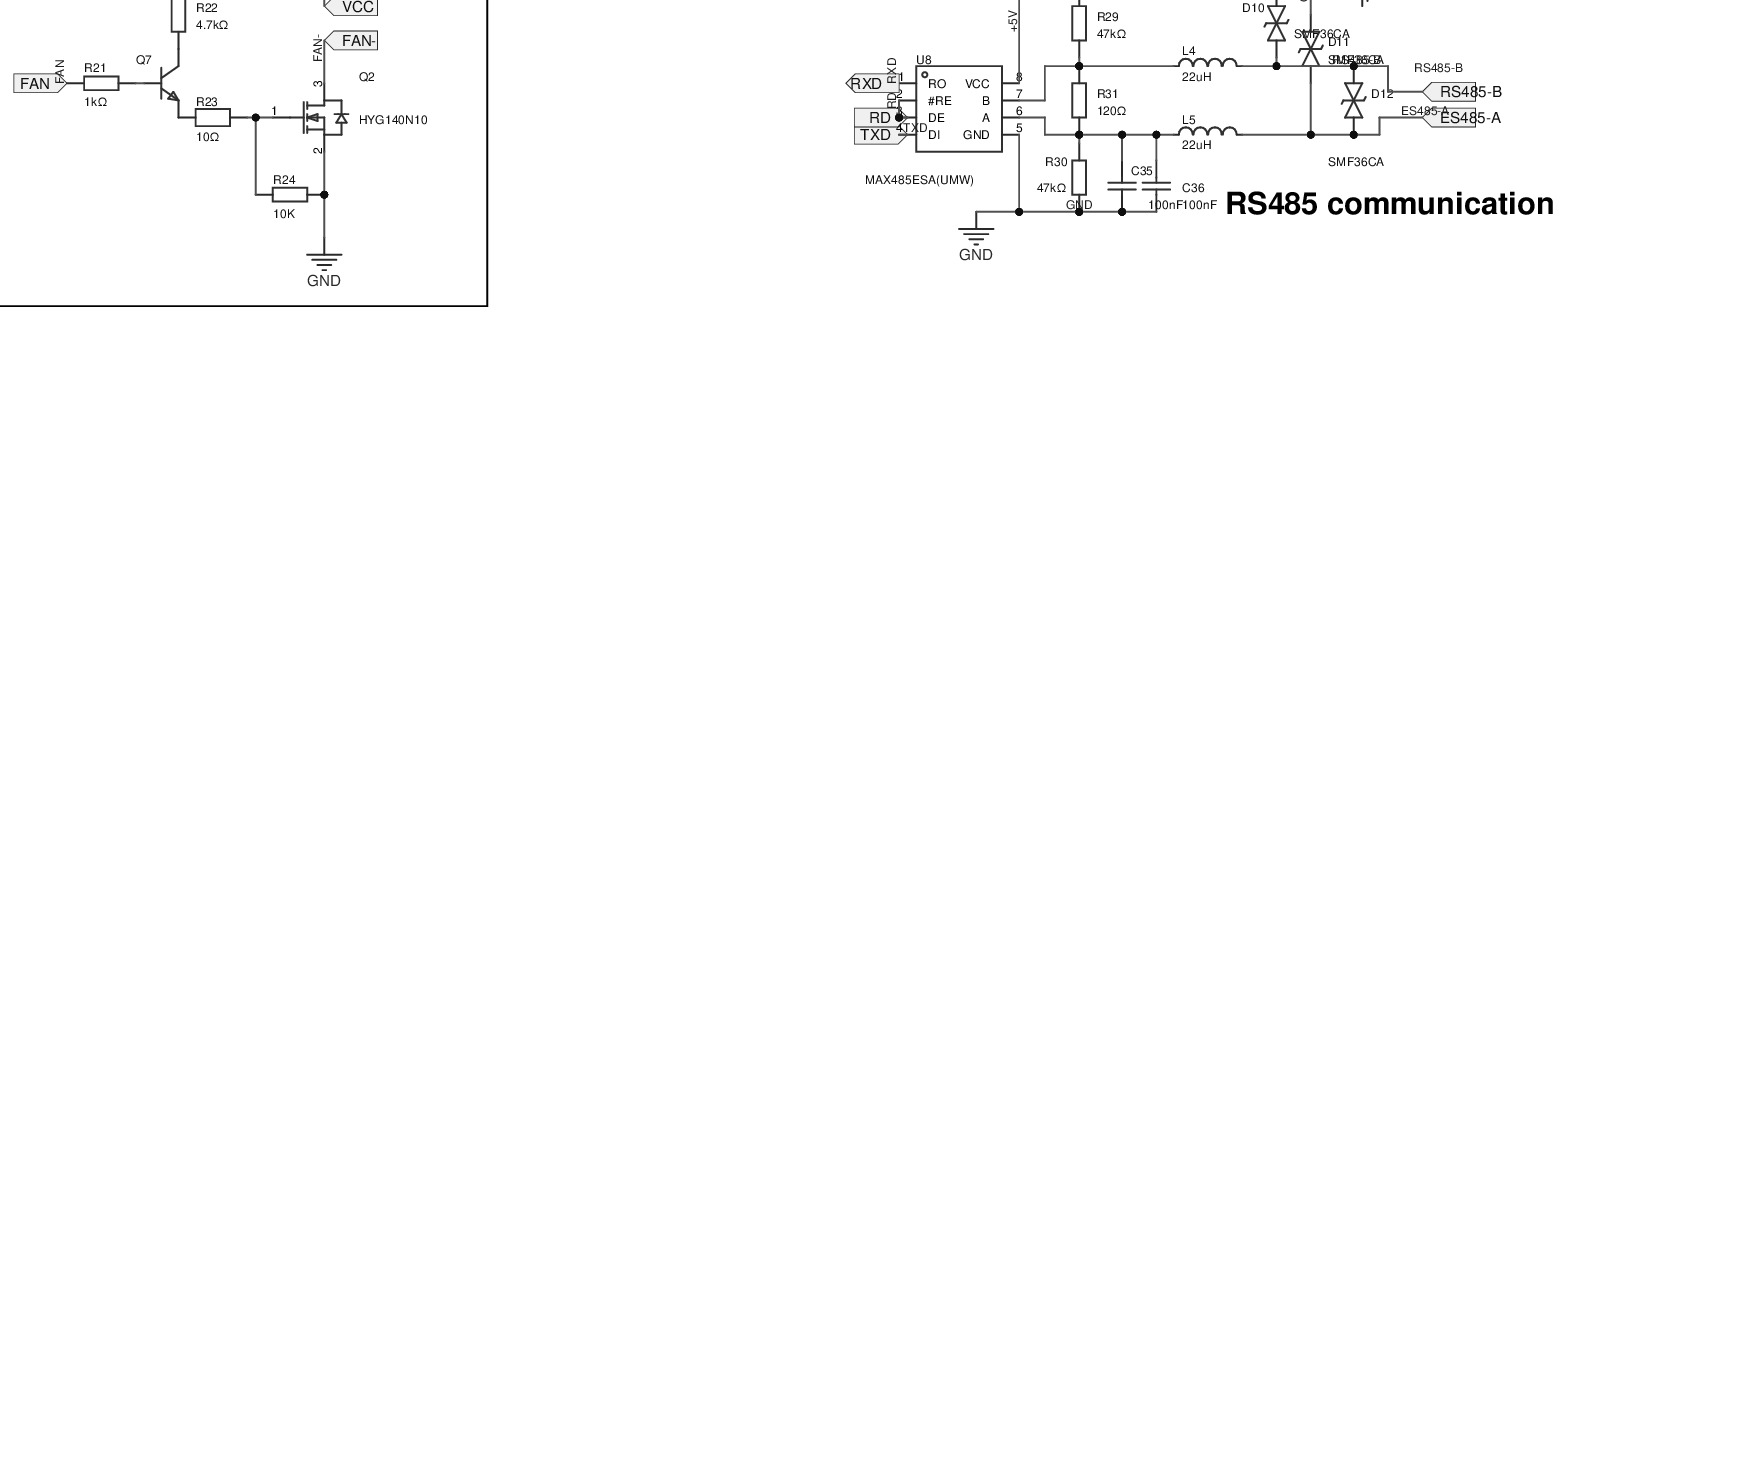
[diagram p0: MISC82093-2.schdoc, bottom right]
# Altium schematic sheet MISC82093-2.schdoc (part 2 of 2)

## Library data of the parts
BUZZER1 = YS-SBZ9650DYB05: Driving method: active (built-in driver circuit); frequency: 2.7kHz; sound pressure (SPL): 80dB;; Manufacturer: Fengming(锋鸣电子); Symbol: YS-SBZ9650DYB05_C409830; AddInBom: yes; ModelId: d9f071f9511e4f7795b1f85db8085480; ModelName: BUZ-SMD_L9.6-W9.6-H5.0; ModelTransform: 393.7,377.952,0,0,0,0,0,0,0; Voltage - Supply: 3V~7V; Device: YS-SBZ9650DYB05; LCSC Part Name: 贴片有源蜂鸣器5V; SupplierPart: C409830; ManufacturerPart: YS-SBZ9650DYB05; Supplier Footprint: SMD,9.6x9.6mm; JLCPCB Part Class: Extended library; Datasheet: https://item.szlcsc.com/datasheet/YS-SBZ9650DYB05/400193.html; Supplier: LCSC; ConvertToPcb: yes; FootprintName: BUZ-SMD_L9.6-W9.6-LS10.0-R; Driver Circuitry: Active (built-in driver circuit); Value: 2.7kHz; Sound Pressure Level(SPL): 80dB; Length: 9.6mm; Width: 9.6mm; Height: 5.3mm
C1 = ECF1KM330F12OTPO: Capacitance: 33uF; tolerance: ±20%; rated voltage: 100V; ripple current: -; equivalent series resistance (ESR): -;; Manufacturer: Yunxing(云星); AddInBom: yes; ModelId: 1445cc51bd6740cbb18bd7447caccb15; ModelTransform: 314.96,315.3537,0,90,0,0,0,0,-196.85; Lifetime: 6000hrs@105℃; Symbol: ECF1KM330F12OTPO; Device: ECF1KM330F12OTPO; LCSC Part Name: 33uF ±20% 100V; SupplierPart: C783507; ManufacturerPart: ECF1KM330F12OTPO; Supplier Footprint: 插件,D8xL12mm; JLCPCB Part Class: Extended library; Datasheet: https://item.szlcsc.com/datasheet/ECF1KM330F12OTPO/837832.html; Supplier: LCSC; ConvertToPcb: yes; FootprintName: CAP-TH_BD8.0-P3.50-D1.0-FD; ModelName: CAP-TH_BD8.0-P3.50-D1.0-FD; Value: 33uF; Tolerance: ±20%; Voltage Rating: 100V; Ripple Current: -; Equivalent Series Resistance(ESR): -; Pin Spacing: -; Diameter: 8mm; Height - Seated (Max): 12mm; Operating Temperature: -40℃~+105℃
C2 C3 = GRM31CL8EL225KE07L: Capacitance: 2.2uF; tolerance: ±10%; rated voltage: 100V; dielectric (temperature coefficient): X8L;; Manufacturer: muRata(村田); AddInBom: yes; ModelId: e4be705b945545a48e666415e3682bd8; ModelName: C1206_L3.2-W1.6-H1.3; ModelTransform: 125.984,62.992,0,0,0,0,0,0,0; Symbol: GRM31CL8EL225KE07L; Device: GRM31CL8EL225KE07L; LCSC Part Name: 2.2uF ±10% 100V; SupplierPart: C5119320; ManufacturerPart: GRM31CL8EL225KE07L; Supplier Footprint: 1206; JLCPCB Part Class: Extended library; Datasheet: https://atta.szlcsc.com/upload/public/pdf/source/20220725/4E0CF642079D992081E87782F4D32939.pdf; Supplier: LCSC; ConvertToPcb: yes; FootprintName: C1206; Value: 2.2uF; Tolerance: ±10%; Voltage Rated: 100V; Temperature Coefficient: X8L
C4 C5 = CAP_1206: Symbol: Capacitance; ConvertToPcb: yes; ModelId: e4be705b945545a48e666415e3682bd8; ModelName: C1206_L3.2-W1.6-H1.3; ModelTransform: 125.984,62.992,0,0,0,0,0,0,0; Device: CAP_1206; AddInBom: yes; Supplier Footprint: 1206; FootprintName: C1206
  C4: Value: 100nF
  C5: Value: 1nF
C6 C9 C10 C13 C14 C16-C19 C23-C26 C30 C35-C37 = CL21B104KBCNNNC: Capacitance: 100nF; tolerance: ±10%; rated voltage: 50V; temperature coefficient: X7R;; Manufacturer: SAMSUNG(三星); AddInBom: yes; ModelId: 1ba041120af144c991958decab20d2410819f05c4eef4c71ace90d822a990e87; ModelName: C0805_L2.0-W1.3-H1.3; ModelTransform: 78.74,51.181,0,0,0,0,0,0.0005,0; Symbol: CL21B104KBCNNNC; Device: CL21B104KBCNNNC; LCSC Part Name: 100nF ±10% 50V; SupplierPart: C1711; ManufacturerPart: CL21B104KBCNNNC; Supplier Footprint: 0805; JLCPCB Part Class: Extended Part; Datasheet: https://item.szlcsc.com/datasheet/CL21B104KBCNNNC/2063.html; Supplier: LCSC; ConvertToPcb: yes; FootprintName: C0805; Value: 100nF; Tolerance: ±10%; Voltage Rating: 50V; Temperature Coefficient: X7R
C7 = GRJ32EC71E226KE11L: Capacitance: 22uF; tolerance: ±10%; rated voltage: 25V; dielectric (temperature coefficient): X7S;; Manufacturer: muRata(村田); AddInBom: yes; ModelId: 833068e7fe044595a6eec77c56179455; ModelName: C1210_L3.2-W2.5-H2.5; ModelTransform: 125.984,98.425,0,0,0,0,0,0,0; Symbol: GRJ32EC71E226KE11L; Device: GRJ32EC71E226KE11L; LCSC Part Name: 22uF ±10% 25V; SupplierPart: C5646747; ManufacturerPart: GRJ32EC71E226KE11L; Supplier Footprint: 1210; JLCPCB Part Class: Extended library; Datasheet: https://atta.szlcsc.com/upload/public/pdf/source/20230811/978878A2AA1A844A6A0C1208031DF55A.pdf; Supplier: LCSC; ConvertToPcb: yes; FootprintName: C1210; Value: 22uF; Tolerance: ±10%; Voltage Rated: 25V; Temperature Coefficient: X7S
C8 C11 = JVS25V100M6X4: Capacitance: 100uF; tolerance: ±20%; rated voltage: 25V; ripple current: 54mA@120Hz;; Manufacturer: JIERR(捷而瑞); AddInBom: yes; Lifetime: 1000hrs@105℃; Symbol: JVS25V100M6X4; Device: JVS25V100M6X4; LCSC Part Name: 100uF ±20% 25V; SupplierPart: C51953404; ManufacturerPart: JVS25V100M6X4; Supplier Footprint: SMD,D6.3xL4.5mm; JLCPCB Part Class: Extended Part; Datasheet: https://item.szlcsc.com/datasheet/JVS25V100M6X4/54681529.html; Supplier: LCSC; ConvertToPcb: yes; FootprintName: CAP-SMD_BD6.3-L6.6-W6.6-LS7.3-FD_JVS25V100M6X4; Value: 100uF; Tolerance: ±20%; Voltage Rating: 25V; Ripple Current: 54mA@120Hz; Diameter: 6.3mm; Height - Seated (Max): 4.5mm; Operating Temperature: -55℃~+105℃
C12 = 35PX470MEFC10X12.5: Capacitance: 470uF; tolerance: ±20%; rated voltage: 35V; ripple current: 525mA@120Hz; equivalent series resistance: -;; Manufacturer: rubycon(红宝石); AddInBom: yes; ModelId: 6ce78ce5315348e095d700085da75e480819f05c4eef4c71ace90d822a990e87; ModelName: CAP-TH_D10.0-H16.0-P5.00; ModelTransform: 394.094,393.72252,0,0,0,0,0,0,-137.795; φD: 10mm; L: 12.5mm; Lifetime @ Temp: 2000hrs@105℃; Symbol: 35PX470MEFC10X12.5; Device: 35PX470MEFC10X12.5; LCSC Part Name: 470uF ±20% 35V; SupplierPart: C127917; ManufacturerPart: 35PX470MEFC10X12.5; Supplier Footprint: 插件,D10xL12.5mm; JLCPCB Part Class: Extended Part; Datasheet: https://atta.szlcsc.com/upload/public/pdf/source/20171026/C136025_15089841766351059112.pdf; Supplier: LCSC; ConvertToPcb: yes; FootprintName: CAP-TH_BD10.0-P5.00-D1.0-FD; Value: 470uF; Tolerance: ±20%; Rated Voltage: 35V; Ripple Current: 525mA@120Hz; Equivalent Series Resistance(ESR): -; Lead Spacing: 5mm; Operating Temperature: -25℃~+105℃
C15 = JVS25V100M6X4: Capacitance: 100uF; tolerance: ±20%; rated voltage: 25V; ripple current: 54mA@120Hz;; Manufacturer: JIERR(捷而瑞); Lifetime: 1000hrs@105℃; AddInBom: yes; Symbol: JVS25V100M6X4; Device: JVS25V100M6X4; LCSC Part Name: 100uF ±20% 25V; Supplier Part: C51953404; Manufacturer Part: JVS25V100M6X4; Supplier Footprint: SMD,D6.3xL4.5mm; JLCPCB Part Class: Extended Part; Datasheet: https://item.szlcsc.com/datasheet/JVS25V100M6X4/54681529.html; Supplier: LCSC; Value: 100uF; Tolerance: ±20%; Voltage Rating: 25V; Ripple Current: 54mA@120Hz; Diameter: 6.3mm; Height - Seated (Max): 4.5mm; Operating Temperature: -55℃~+105℃; ConvertToPcb: yes; FootprintName: CAP-SMD_BD6.3-L6.6-W6.6-LS7.3-FD_JVS25V100M6X4
C20 = CAP_0805: Symbol: Capacitance; ConvertToPcb: yes; ModelId: 1ba041120af144c991958decab20d241; ModelName: C0805_L2.0-W1.3-H1.3; ModelTransform: 78.74,51.181,0,0,0,0,0,0.0005,0; Value: 0.1uF; Device: CAP_0805; AddInBom: yes; Supplier Footprint: 0805; FootprintName: C0805
C21 C22 = CL21C220JBANNNC: Capacitance: 22pF; tolerance: ±5%; rated voltage: 50V; temperature coefficient: C0G;; Manufacturer: SAMSUNG(三星); AddInBom: yes; ModelId: 1ba041120af144c991958decab20d2410819f05c4eef4c71ace90d822a990e87; ModelName: C0805_L2.0-W1.3-H1.3; ModelTransform: 78.74,51.181,0,0,0,0,0,0.0005,0; Symbol: CL21C220JBANNNC; Device: CL21C220JBANNNC; LCSC Part Name: 22pF ±5% 50V; SupplierPart: C1804; ManufacturerPart: CL21C220JBANNNC; Supplier Footprint: 0805; JLCPCB Part Class: Basic Part; Datasheet: https://item.szlcsc.com/datasheet/CL21C220JBANNNC/2156.html; Supplier: LCSC; ConvertToPcb: yes; FootprintName: C0805; Value: 22pF; Tolerance: ±5%; Voltage Rating: 50V; Temperature Coefficient: C0G
C27-C29 = CL21C101JBANNNC: Capacitance: 100pF; tolerance: ±5%; rated voltage: 50V; temperature coefficient: C0G;; Manufacturer: SAMSUNG(三星); AddInBom: yes; ModelId: 1ba041120af144c991958decab20d2410819f05c4eef4c71ace90d822a990e87; ModelName: C0805_L2.0-W1.3-H1.3; ModelTransform: 78.74,51.181,0,0,0,0,0,0.0005,0; Symbol: CL21C101JBANNNC; Device: CL21C101JBANNNC; LCSC Part Name: 100pF ±5% 50V; SupplierPart: C1790; ManufacturerPart: CL21C101JBANNNC; Supplier Footprint: 0805; JLCPCB Part Class: Basic Part; Datasheet: https://item.szlcsc.com/datasheet/CL21C101JBANNNC/2142.html; Supplier: LCSC; ConvertToPcb: yes; FootprintName: C0805; Value: 100pF; Tolerance: ±5%; Voltage Rating: 50V; Temperature Coefficient: C0G
C31-C34 = 0805X5R106K500NT: Capacitance: 10uF; tolerance: ±10%; rated voltage: 50V; temperature coefficient: X5R;; Manufacturer: AIDE(爱迪电容); AddInBom: yes; ModelId: 1ba041120af144c991958decab20d241; ModelName: C0805_L2.0-W1.3-H1.3; ModelTransform: 78.74,51.181,0,0,0,0,0,0.0005,0; Symbol: 0805X5R106K500NT; Device: 0805X5R106K500NT; LCSC Part Name: 10uF ±10% 50V; ManufacturerPart: 0805X5R106K500NT; Supplier Footprint: 0805; JLCPCB Part Class: Extended library; Datasheet: https://atta.szlcsc.com/upload/public/pdf/source/20250425/87F0660DBF100371164E520B4251C19E.pdf; Supplier: LCSC; ConvertToPcb: yes; FootprintName: C0805; Tolerance: ±10%; Voltage Rating: 50V; Temperature Coefficient: X5R
  C31 C33: SupplierPart: C48579582; Value: 10uF
  C32 C34: Value: 1uF
C38 C39 = GRJ32EC71E226KE11L: Capacitance: 22uF; tolerance: ±10%; rated voltage: 25V; dielectric (temperature coefficient): X7S;; Manufacturer: muRata(村田); 3D Model: 833068e7fe044595a6eec77c56179455; 3D Model Transform: 125.984,98.425,0,0,0,0,0,0,0; AddInBom: yes; ModelName: C1210_L3.2-W2.5-H2.5; Symbol: GRJ32EC71E226KE11L; Device: GRJ32EC71E226KE11L; LCSC Part Name: 22uF ±10% 25V; Supplier Part: C5646747; Manufacturer Part: GRJ32EC71E226KE11L; Supplier Footprint: 1210; JLCPCB Part Class: Extended library; Datasheet: https://atta.szlcsc.com/upload/public/pdf/source/20230811/978878A2AA1A844A6A0C1208031DF55A.pdf; Supplier: LCSC; Value: 22uF; Tolerance: ±10%; Voltage Rated: 25V; Temperature Coefficient: X7S; ConvertToPcb: yes; FootprintName: C1210
C40 = CL21B104KBCNNNC: Capacitance: 100nF; tolerance: ±10%; rated voltage: 50V; temperature coefficient: X7R;; Manufacturer: SAMSUNG(三星); 3D Model: 1ba041120af144c991958decab20d2410819f05c4eef4c71ace90d822a990e87; 3D Model Transform: 78.74,51.181,0,0,0,0,0,0.0005,0; AddInBom: yes; ModelName: C0805_L2.0-W1.3-H1.3; Symbol: CL21B104KBCNNNC; Device: CL21B104KBCNNNC; LCSC Part Name: 100nF ±10% 50V; Supplier Part: C1711; Manufacturer Part: CL21B104KBCNNNC; Supplier Footprint: 0805; JLCPCB Part Class: Extended Part; Datasheet: https://item.szlcsc.com/datasheet/CL21B104KBCNNNC/2063.html; Supplier: LCSC; Value: 100nF; Tolerance: ±10%; Voltage Rating: 50V; Temperature Coefficient: X7R; ConvertToPcb: yes; FootprintName: C0805
C41 = CL21B102KBCNNNC: Capacitance: 1nF; tolerance: ±10%; rated voltage: 50V; temperature coefficient: X7R;; Manufacturer: SAMSUNG(三星); AddInBom: yes; ModelId: 1ba041120af144c991958decab20d2410819f05c4eef4c71ace90d822a990e87; ModelName: C0805_L2.0-W1.3-H1.3; ModelTransform: 78.74,51.181,0,0,0,0,0,0.0005,0; Symbol: CL21B102KBCNNNC; Device: CL21B102KBCNNNC; LCSC Part Name: 1nF ±10% 50V; SupplierPart: C46653; ManufacturerPart: CL21B102KBCNNNC; Supplier Footprint: 0805; JLCPCB Part Class: Basic Part; Datasheet: https://item.szlcsc.com/datasheet/CL21B102KBCNNNC/47657.html; Supplier: LCSC; ConvertToPcb: yes; FootprintName: C0805; Value: 1nF; Tolerance: ±10%; Voltage Rating: 50V; Temperature Coefficient: X7R
D1 = US2M-TP: Diode configuration: -; forward voltage (Vf): 1.7V@2A; DC reverse voltage (Vr): 1kV; rectified current: 2A; reverse recovery time (Trr): 100ns;; Manufacturer: MCC(美微科); AddInBom: yes; ModelId: 5e8926c661484ff2a35b83e5ae62aeb90819f05c4eef4c71ace90d822a990e87; ModelTransform: 212.598,141.732,0,0,0,0,0,0,0; Reverse Leakage Current (Ir): 5uA@1kV; Operating Junction Temperature Range: -50℃~+150℃@(Ta); Non-Repetitive Peak Forward Surge Current: 50A; Symbol: US2M-TP; Device: US2M-TP; LCSC Part Name: 耐压:1kV 电流:2A 反向恢复时间：100ns; SupplierPart: C138791; ManufacturerPart: US2M-TP; Supplier Footprint: DO-214AA(SMB); JLCPCB Part Class: Extended Part; Datasheet: https://item.szlcsc.com/datasheet/US2M-TP/150112.html; Supplier: LCSC; ConvertToPcb: yes; FootprintName: SMB_L4.6-W3.6-LS5.3-RD; ModelName: SMB_L4.6-W3.6-LS5.3-RD; Diode Configuration: -; Voltage - Forward(Vf@If): 1.7V@2A; Voltage - DC Reverse(Vr): 1kV; Current - Rectified: 2A; Reverse Recovery Time (trr): 100ns
D2 D3 = SS34_C8678: Diode configuration: single; forward voltage (Vf): 550mV@3A; DC reverse voltage (Vr): 40V; rectified current: 3A;; Manufacturer: MDD(辰达半导体); 3D Model: e3551acb3c5a4975a5e9d36087fe1fa2; 3D Model Transform: 185.039,102.362,0,0,0,0,0,0,0; Reverse Leakage Current (Ir): 500uA@40V; Operating Junction Temperature Range: -55℃~+125℃; AddInBom: yes; Symbol: SS34_C8678; Device: SS34_C8678; LCSC Part Name: 电压:40V 电流:3A; Supplier Part: C8678; Manufacturer Part: SS34; Supplier Footprint: SMA(DO-214AC); JLCPCB Part Class: Basic library; Datasheet: https://item.szlcsc.com/datasheet/SS34/9178.html; Supplier: LCSC; Diode Configuration: Single; Voltage - Forward(Vf@If): 550mV@3A; Voltage - DC Reverse(Vr): 40V; Current - Rectified: 3A; ConvertToPcb: yes; FootprintName: SMA_L4.3-W2.6-LS5.2-RD; ModelName: SMA_L4.3-W2.6-LS5.2-RD
D4 D5 = MUR160SB: Diode configuration: single; forward voltage (Vf): 1.3V@1A; DC reverse voltage (Vr): 600V; rectified current: 1A; reverse recovery time (Trr): 50ns;; Manufacturer: AM(安美); AddInBom: yes; ModelId: 892cc756ed79448ab4afad0e5bfcdfa6; ModelTransform: 212.598,141.732,0,0,0,0,0,0,0; Symbol: MUR160SB; Device: MUR160SB; LCSC Part Name: MUR160SB; SupplierPart: C18336927; ManufacturerPart: MUR160SB; Supplier Footprint: SMB; JLCPCB Part Class: Extended library; Datasheet: https://atta.szlcsc.com/upload/public/pdf/source/20231016/5AD88B7244EB32ADD8FE31282D3178E2.pdf; Supplier: LCSC; ConvertToPcb: yes; FootprintName: SMB_L4.6-W3.6-LS5.3-RD; ModelName: SMB_L4.6-W3.6-LS5.3-RD; Diode Configuration: Single; Voltage - Forward(Vf@If): 1.3V@1A; Voltage - DC Reverse(Vr): 600V; Current - Rectified: 1A; Reverse Recovery Time (trr): 50ns
D6-D9 = RB160M-90: Forward voltage (Vf): 750mV@1.0A; DC reverse voltage (Vr): 90V; rectified current: 1A;; Manufacturer: TECH PUBLIC(台舟); AddInBom: yes; ModelId: 86f9151e155e4fe2af0c4f2e0a80302e; ModelName: SOD-123FL_L2.8-W1.8-H1.1-LS3.6; ModelTransform: 141.732,70.866,0,180,0,0,0,0,0; Reverse Leakage Current (Ir): 100uA@100V; Operating Junction Temperature Range: -55℃~+150℃; Non-Repetitive Peak Forward Surge Current: 50A; Symbol: RB160M-90; Device: RB160M-90; LCSC Part Name: 电压:90V 电流:1A; SupplierPart: C7603322; ManufacturerPart: RB160M-90; Supplier Footprint: SOD-123FL; JLCPCB Part Class: Extended library; Datasheet: https://item.szlcsc.com/datasheet/RB160M-90/8728828.html; Supplier: LCSC; ConvertToPcb: yes; FootprintName: SOD-123FL_L2.7-W1.8-LS3.7-RD; Voltage - Forward(Vf@If): 750mV@1.0A; Voltage - DC Reverse(Vr): 90V; Current - Rectified: 1A
D10-D12 = SMF36CA_C435502: Polarity: bidirectional; reverse standoff voltage (Vrwm): 36V; clamping voltage: 58.1V; peak pulse current (Ipp): 3.5A; peak pulse power (Ppp): 200W@10/1000us; breakdown voltage: 40V;; Manufacturer: AnBon(安邦); 3D Model: 8576f175c34f41329e79954aa68cc529; 3D Model Transform: 145.669,70.866,0,0,0,0,0,0,0; Reverse Leakage Current (Ir): 5uA; Number of Channels: Single channel; Type: TVS; AddInBom: yes; Symbol: SMF36CA_C435502; Device: SMF36CA_C435502; LCSC Part Name: SMF36CA; Supplier Part: C435502; Manufacturer Part: SMF36CA; Supplier Footprint: SOD-123; JLCPCB Part Class: Extended library; Datasheet: https://item.szlcsc.com/datasheet/SMF36CA/432840.html; Supplier: LCSC; Polarity: Bidirectional; Reverse Stand-Off Voltage (Vrwm): 36V; Clamping Voltage: 58.1V; Peak Pulse Current (Ipp): 3.5A; Peak Pulse Power Dissipation (Ppp): 200W@10/1000us; Voltage - Breakdown: 40V; Operating Temperature: -55℃~+150℃; ConvertToPcb: yes; FootprintName: SOD-123_L2.7-W1.8-LS3.7-BI; ModelName: SOD-123_L2.7-W1.8-LS3.7-BI
L1 = FXL1040-330-M: Inductance: 33uH; tolerance: ±20%; rated current: 4.4A; saturation current (Isat): 5A; type: molded inductor;; Manufacturer: cjiang(长江微电); 3D Model: c9cd86c9f1ef4d748cb9537bf0f243250819f05c4eef4c71ace90d822a990e87; 3D Model Transform: 452.755,393.7,0,0,0,0,0,0,0; DC Resistance(DCR): 92mΩ; AddInBom: yes; ModelName: IND-SMD_L11.5-W10.0-H3.8_FXL1040; Symbol: FXL1040-330-M; Device: FXL1040-330-M; LCSC Part Name: 33uH ±20% 5A; Supplier Part: C475918; Manufacturer Part: FXL1040-330-M; Supplier Footprint: SMD,11.5x10mm; JLCPCB Part Class: Extended Part; Datasheet: https://item.szlcsc.com/datasheet/FXL1040-330-M/482451.html; Supplier: LCSC; Value: 33uH; Tolerance: ±20%; Current Rating: 4.4A; Current - Saturation(Isat): 5A; Type: Molded inductor; ConvertToPcb: yes; FootprintName: IND-SMD_L11.5-W10.0_FXL1040
L2 L3 = PSPMAA0605H-680M-IGF: Inductance: 68uH; tolerance: ±20%; rated current: 1.5A; saturation current (Isat): 2A; type: -;; Manufacturer: PROD(谱罗德); AddInBom: yes; ModelId: 42305e89796f47b49312a685ea93d4940819f05c4eef4c71ace90d822a990e87; ModelName: IND-SMD_L7.1-W6.6-H5.0; ModelTransform: 275.59,259.88137,0,0,0,0,0,-0.551,0; DC Resistance(DCR): 256mΩ; Symbol: PSPMAA0605H-680M-IGF; Device: PSPMAA0605H-680M-IGF; LCSC Part Name: 68uH ±20% 2A; SupplierPart: C2983094; ManufacturerPart: PSPMAA0605H-680M-IGF; Supplier Footprint: SMD,7.1x6.6mm; JLCPCB Part Class: Extended Part; Datasheet: https://item.szlcsc.com/datasheet/PSPMAA0605H-680M-IGF/3416346.html; Supplier: LCSC; ConvertToPcb: yes; FootprintName: IND-SMD_L7.1-W6.6_H5.0; Value: 68uH; Tolerance: ±20%; Current Rating: 1.5A; Current - Saturation(Isat): 2A; Type: -; Ratings: -
L4 L5 = SCL3216T220KSP: Inductance: 22uH; tolerance: ±10%; rated current: 5mA; saturation current (Isat): -; DC resistance (DCR): 900mΩ;; Manufacturer: Sunltech(顺磁); AddInBom: yes; ModelId: 85bdab7b3d4c4074b81d208eb5e865b30819f05c4eef4c71ace90d822a990e87; ModelName: L1206_L3.2-W1.6-H1.1; ModelTransform: 125.984,62.835,0,0,0,0,0,0,0; Symbol: SCL3216T220KSP; Device: SCL3216T220KSP; LCSC Part Name: 22uH ±10%; SupplierPart: C412019; ManufacturerPart: SCL3216T220KSP; Supplier Footprint: 1206; JLCPCB Part Class: Extended Part; Datasheet: https://item.szlcsc.com/datasheet/SCL3216T220KSP/403512.html; Supplier: LCSC; ConvertToPcb: yes; FootprintName: L1206; Value: 22uH; Tolerance: ±10%; Current Rating: 5mA; Current - Saturation (Isat): -; DC Resistance(DCR): 900mΩ; Q @ Frequency: -; Frequency - Self Resonant: -; Ratings: -
LED1-LED4 = 3mmFIR: AddInBom: yes; ModelId: a497c992633541038a38947cdc58012f; ModelName: LED-TH-3mm_R; ModelTransform: 141.274,153.327,0,0,0,0,-5.984,0,-137.795; Symbol: 3MMFIR; Device: 3mmFIR; LCSC Part Name: 3mmFIR; SupplierPart: C9900095018; ManufacturerPart: 3mmFIR; Supplier Footprint: LED-TH_LED-3MM_RED; JLCPCB Part Class: Extended library; Supplier: LCSC; ConvertToPcb: yes; FootprintName: LED-TH_BD3.0-P2.54-FD
LED5 = SP420361N: Number of digits: 3; character size (inch): 0.36; color: red; LED polarity: common cathode;; Manufacturer: ARKLED(方舟); AddInBom: yes; ModelId: 75b7188ef1934ceeb211c7922abf127e0819f05c4eef4c71ace90d822a990e87; ModelTransform: 885.825,551.5737,0,90,0,0,0,0,-196.85; Number of Characters: 3 digits; Digit/Alpha Size(inch): 0.36; Symbol: SP420361N; Device: SP420361N; LCSC Part Name: 3位0.36英寸红色数码管 共阴极; SupplierPart: C98927; ManufacturerPart: SP420361N; Supplier Footprint: 插件; JLCPCB Part Class: Extended Part; Datasheet: https://item.szlcsc.com/datasheet/SP420361N/100139.html; Supplier: LCSC; ConvertToPcb: yes; FootprintName: LED-SEG-TH_SP420361N; ModelName: LED-SEG-TH_SP420361N; Illumination Color: Red; LED Polarity: Common cathode
Q1 = SS8050(RANGE:200-350)_C2150: Transistor type: NPN; collector current (Ic): 1.5A; collector-emitter breakdown voltage (Vceo): 25V; power (Pd): 300mW; DC current gain (hFE@Ic,Vce): 200@800mA,1V;; Manufacturer: CJ(江苏长电/长晶); Symbol: SS8050_C2150; AddInBom: yes; ModelId: c62791f0466c4ae2a892c056b845b0ca; ModelName: SOT-23-3P_L2.9-W1.3-H1.0-LS2.4-P0.95; ModelTransform: 98.425,114.173,0,180,0,0,0.0005,-0.0005,0; Transition Frequency (fT): 100MHz; Collector Cut-Off Current (Icbo): 100nA; Collector-Emitter Saturation Voltage (VCE(sat)@Ic,Ib): 500mV@800mA,80mA; Device: SS8050(RANGE:200-350)_C2150; LCSC Part Name: NPN 电流:1.5A 耐压:25V hfe=200~350; SupplierPart: C2150; ManufacturerPart: SS8050(RANGE:200-350); Supplier Footprint: SOT-23; JLCPCB Part Class: Basic library; Datasheet: https://atta.szlcsc.com/upload/public/pdf/source/20230322/AEE86F4B043774EFF80CAEA14A37D9E9.pdf; Supplier: LCSC; ConvertToPcb: yes; FootprintName: SOT-23-3_L2.9-W1.3-P1.90-LS2.4-BR; Transistor Type: NPN; Collector Current (Ic): 1.5A; Collector-Emitter Breakdown Voltage (Vceo): 25V; Power Dissipation (Pd): 300mW; DC Current Gain (hFE@Ic,Vce): 200@800mA,1V; Operating Temperature: -55℃~+150℃
Q2 = NCE0140K2-VB: Type: 1 N-channel; drain-source voltage (Vdss): 100V; continuous drain current (Id): 45A; on-resistance (RDS(on)@Vgs,Id): -; power (Pd): 3W; threshold voltage (Vgs(th)@Id): 2.5V@250uA;; Manufacturer: VBsemi(微碧半导体); 3D Model: 002f14490d3e47dc80a93c97f5a1e7bb; 3D Model Transform: 385.5088,255.905,0,0,0,0,-33.661,0,0; Total Gate Charge (Qg@Vgs): 38nC@10V; Input Capacitance (Ciss@Vds): 2.4nF@50V; Reverse Transfer Capacitance (Crss@Vds): 80pF@50V; AddInBom: yes; Symbol: NCE0140K2-VB; Device: NCE0140K2-VB; Manufacturer Part: HYG140N10; LCSC Part Name: 1个N沟道 耐压:100V 电流:45A; Supplier Part: C7463473; Supplier Footprint: TO-252; JLCPCB Part Class: Extended library; Datasheet: https://atta.szlcsc.com/upload/public/pdf/source/20240821/DCE0DDCDA6E2F6C426FEF52E9193F584.pdf; Supplier: LCSC; Drain Source Voltage (Vdss): 100V; Continuous Drain Current (Id): 45A; Drain Source On Resistance (RDS(on)@Vgs,Id): -; Power Dissipation (Pd): 3W; Gate Threshold Voltage (Vgs(th)@Id): 2.5V@250uA; Operating Temperature: -55℃~+175℃; ConvertToPcb: yes; FootprintName: TO-252-3_L6.6-W6.1-P4.58-LS10.1-BR; ModelName: TO-252-3_L6.6-W6.1-P4.58-LS10.1-BR
Q3-Q6 = HYG025N06LS1B: Quantity: 1 N-channel; drain-source voltage (Vdss): 60V; continuous drain current (Id): 160A; on-resistance (RDS(on)): 3.3mΩ@10V; power dissipation (Pd): 125W; threshold voltage (Vgs(th)): 3V@250uA;; Manufacturer: HUAYI(华羿微); AddInBom: yes; ModelId: e74d9d1f92e14ef38b829eb45550a5f50819f05c4eef4c71ace90d822a990e87; ModelTransform: 399.999,594.487,0,90,0,0,-25.236,0,0; Gate Charge(Qg): 58.3nC@10V; Input Capacitance(Ciss): 3.915nF; Reverse Transfer Capacitance (Crss@Vds): 10.2pF; Output Capacitance(Coss): 1.31nF; Symbol: HYG025N06LS1B; Device: HYG025N06LS1B; LCSC Part Name: 1个N沟道 耐压:60V 电流:160A; SupplierPart: C2836680; ManufacturerPart: HYG025N06LS1B; Supplier Footprint: TO-263-2L; JLCPCB Part Class: Extended Part; Datasheet: https://item.szlcsc.com/datasheet/HYG025N06LS1B/3004274.html; Supplier: LCSC; ConvertToPcb: yes; FootprintName: TO-263-2_L10.2-W8.7-P5.08-LS15.1-BR; ModelName: TO-263-2_L10.2-W8.7-P5.08-LS15.1-BR; Number: 1 N-channel; Drain to Source Voltage: 60V; Current - Continuous Drain(Id): 160A; RDS(on): 3.3mΩ@10V; Pd - Power Dissipation: 125W; Gate Threshold Voltage (Vgs(th)): 3V@250uA; Operating Temperature: -55℃~+175℃; Type: N-channel
Q7 = SS8050(RANGE:200-350)_C2150: Transistor type: NPN; collector current (Ic): 1.5A; collector-emitter breakdown voltage (Vceo): 25V; power (Pd): 300mW; DC current gain (hFE@Ic,Vce): 200@800mA,1V;; Manufacturer: CJ(江苏长电/长晶); Symbol: SS8050_C2150; 3D Model: c62791f0466c4ae2a892c056b845b0ca; 3D Model Transform: 98.425,114.173,0,180,0,0,0.0005,-0.0005,0; Transition Frequency (fT): 100MHz; Collector Cut-Off Current (Icbo): 100nA; Collector-Emitter Saturation Voltage (VCE(sat)@Ic,Ib): 500mV@800mA,80mA; AddInBom: yes; ModelName: SOT-23-3P_L2.9-W1.3-H1.0-LS2.4-P0.95; Device: SS8050(RANGE:200-350)_C2150; LCSC Part Name: NPN 电流:1.5A 耐压:25V hfe=200~350; Supplier Part: C2150; Manufacturer Part: SS8050(RANGE:200-350); Supplier Footprint: SOT-23; JLCPCB Part Class: Basic library; Datasheet: https://atta.szlcsc.com/upload/public/pdf/source/20230322/AEE86F4B043774EFF80CAEA14A37D9E9.pdf; Supplier: LCSC; Transistor Type: NPN; Collector Current (Ic): 1.5A; Collector-Emitter Breakdown Voltage (Vceo): 25V; Power Dissipation (Pd): 300mW; DC Current Gain (hFE@Ic,Vce): 200@800mA,1V; Operating Temperature: -55℃~+150℃; ConvertToPcb: yes; FootprintName: SOT-23-3_L2.9-W1.3-P1.90-LS2.4-BR
R1 = CR0805-FX-6492ELF: Resistor type: thick film resistor; resistance: 64.9kΩ; tolerance: ±1%; power: 125mW; operating voltage: 150V; temperature coefficient: ±100ppm/℃;; Manufacturer: BOURNS; AddInBom: yes; ModelId: 37a81e68749a4138bd2dfa6897b24b850819f05c4eef4c71ace90d822a990e87; ModelName: R0805_L2.0-W1.3-H0.6; ModelTransform: 78.74,51.181,0,0,0,0,0,-0.0005,0; Symbol: CR0805-FX-6492ELF; Device: CR0805-FX-6492ELF; LCSC Part Name: 厚膜电阻 64.9kΩ ±1% 125mW; SupplierPart: C204250; ManufacturerPart: CR0805-FX-6492ELF; Supplier Footprint: 0805; JLCPCB Part Class: Extended Part; Datasheet: https://item.szlcsc.com/datasheet/CR0805-FX-6492ELF/205732.html; Supplier: LCSC; ConvertToPcb: yes; FootprintName: R0805; Type: Thick film resistor; Value: 64.9kΩ; Tolerance: ±1%; Power(Watts): 125mW; Voltage-Supply(Max): 150V; Temperature Coefficient: ±100ppm/℃; Operating Temperature: -55℃~+155℃
R2 = CR0805-10W-104JT: Resistor type: thick film resistor; resistance: 100kΩ; tolerance: ±5%; power: 100mW; temperature coefficient: ±200ppm/℃;; Manufacturer: Venkel; AddInBom: yes; ModelId: 37a81e68749a4138bd2dfa6897b24b85; ModelName: R0805_L2.0-W1.3-H0.6; ModelTransform: 78.74,51.181,0,0,0,0,0,-0.0005,0; Symbol: CR0805-10W-104JT; Device: CR0805-10W-104JT; LCSC Part Name: 厚膜电阻 100kΩ ±5% 100mW; SupplierPart: C3971088; ManufacturerPart: CR0805-10W-104JT; Supplier Footprint: 0805; Datasheet: https://atta.szlcsc.com/upload/public/pdf/source/231023/CR-Series-b7b6a911051dbc65fedbe53708428339.pdf; Supplier: LCSC; ConvertToPcb: yes; FootprintName: R0805; Type: Thick film resistor; Value: 100kΩ; Tolerance: ±5%; Power(Watts): 100mW; Temperature Coefficient: ±200ppm/℃; Operating Temperature: -55℃~+155℃
R3 = RCA0524K9FLF: Resistance: 24.9kΩ; tolerance: ±1%; power: 125mW;; Manufacturer: HKR(香港电阻); AddInBom: yes; ModelId: 37a81e68749a4138bd2dfa6897b24b85; ModelName: R0805_L2.0-W1.3-H0.6; ModelTransform: 78.74,51.181,0,0,0,0,0,-0.0005,0; Value: 9.09kΩ; Symbol: RCA0524K9FLF; Device: RCA0524K9FLF; LCSC Part Name: 24.9kΩ ±1% 125mW; ManufacturerPart: RCA0524K9FLF; Supplier Footprint: 0805; Datasheet: https://atta.szlcsc.com/upload/public/pdf/source/20240327/626E23E3B2A799D2C85303DE2C37BB2A.pdf; Supplier: LCSC; ConvertToPcb: yes; FootprintName: R0805; Tolerance: ±1%; Power(Watts): 125mW
R4 R25-R27 = Res_0805: Symbol: Resistor; ConvertToPcb: yes; ModelId: 37a81e68749a4138bd2dfa6897b24b85; ModelName: R0805_L2.0-W1.3-H0.6; ModelTransform: 78.74,51.181,0,0,0,0,0,-0.0005,0; Device: Res_0805; AddInBom: yes; Supplier Footprint: 0805; Value: 10K; FootprintName: R0805
R5 = 0805W8F1004T5E: Resistor type: thick film resistor; resistance: 1MΩ; tolerance: ±1%; power: 125mW; max operating voltage: 150V; temperature coefficient: ±100ppm/℃;; Manufacturer: UNI-ROYAL(厚声); AddInBom: yes; ModelId: 37a81e68749a4138bd2dfa6897b24b850819f05c4eef4c71ace90d822a990e87; ModelName: R0805_L2.0-W1.3-H0.6; ModelTransform: 78.74,51.181,0,0,0,0,0,-0.0005,0; Symbol: 0805W8F1004T5E; Device: 0805W8F1004T5E; LCSC Part Name: 1MΩ ±1% 125mW 厚膜电阻; SupplierPart: C17514; ManufacturerPart: 0805W8F1004T5E; Supplier Footprint: 0805; JLCPCB Part Class: Basic Part; Datasheet: https://atta.szlcsc.com/upload/public/pdf/source/20200306/C422600_1E6D84923E4A46A82E41ADD87F860B5C.pdf; Supplier: LCSC; ConvertToPcb: yes; FootprintName: R0805; Type: Thick film resistor; Value: 1MΩ; Tolerance: ±1%; Power(Watts): 125mW; Overload Voltage (Max): 150V; Temperature Coefficient: ±100ppm/℃; Operating Temperature Range: -55℃~+155℃
R6-R9 = 0805W8F1000T5E: Resistor type: thick film resistor; resistance: 100Ω; tolerance: ±1%; power: 125mW; max operating voltage: 150V; temperature coefficient: ±100ppm/℃;; Manufacturer: UNI-ROYAL(厚声); AddInBom: yes; ModelId: 37a81e68749a4138bd2dfa6897b24b850819f05c4eef4c71ace90d822a990e87; ModelName: R0805_L2.0-W1.3-H0.6; ModelTransform: 78.74,51.181,0,0,0,0,0,-0.0005,0; Symbol: 0805W8F1000T5E; Device: 0805W8F1000T5E; LCSC Part Name: 100Ω ±1% 125mW 厚膜电阻; SupplierPart: C17408; ManufacturerPart: 0805W8F1000T5E; Supplier Footprint: 0805; JLCPCB Part Class: Basic Part; Datasheet: https://atta.szlcsc.com/upload/public/pdf/source/20200306/C422600_1E6D84923E4A46A82E41ADD87F860B5C.pdf; Supplier: LCSC; ConvertToPcb: yes; FootprintName: R0805; Type: Thick film resistor; Value: 100Ω; Tolerance: ±1%; Power(Watts): 125mW; Overload Voltage (Max): 150V; Temperature Coefficient: ±100ppm/℃; Operating Temperature Range: -55℃~+155℃
R10-R13 = 0805W8J0472T5E: Resistor type: thick film resistor; resistance: 4.7kΩ; tolerance: ±5%; power: 125mW; operating voltage: 150V; temperature coefficient: ±100ppm/℃;; Manufacturer: UNI-ROYAL(厚声); AddInBom: yes; ModelId: 37a81e68749a4138bd2dfa6897b24b850819f05c4eef4c71ace90d822a990e87; ModelName: R0805_L2.0-W1.3-H0.6; ModelTransform: 78.74,51.181,0,0,0,0,0,-0.0005,0; Symbol: 0805W8J0472T5E; Device: 0805W8J0472T5E; LCSC Part Name: 4.7kΩ ±5% 125mW 厚膜电阻; SupplierPart: C26022; ManufacturerPart: 0805W8J0472T5E; Supplier Footprint: 0805; JLCPCB Part Class: Extended Part; Datasheet: https://item.szlcsc.com/datasheet/0805W8J0472T5E/26765.html; Supplier: LCSC; ConvertToPcb: yes; FootprintName: R0805; Type: Thick film resistor; Value: 4.7kΩ; Tolerance: ±5%; Power(Watts): 125mW; Voltage-Supply(Max): 150V; Temperature Coefficient: ±100ppm/℃; Operating Temperature: -55℃~+155℃
R14-R16 R24 = Res_0805: Symbol: Resistor; 3D Model: 37a81e68749a4138bd2dfa6897b24b85; 3D Model Transform: 78.74,51.181,0,0,0,0,0,-0.0005,0; ConvertToPcb: yes; ModelName: R0805_L2.0-W1.3-H0.6; Device: Res_0805; Supplier Footprint: 0805; Value: 10K; AddInBom: yes; FootprintName: R0805
R17-R20 = CRCW080510R0FKEAC: Resistor type: thick film resistor; resistance: 10Ω; tolerance: ±1%; power: 125mW; temperature coefficient: ±100ppm/℃;; Manufacturer: VISHAY(威世); AddInBom: yes; ModelId: 37a81e68749a4138bd2dfa6897b24b85; ModelName: R0805_L2.0-W1.3-H0.6; ModelTransform: 78.74,51.181,0,0,0,0,0,-0.0005,0; Symbol: CRCW080510R0FKEAC; Device: CRCW080510R0FKEAC; LCSC Part Name: 厚膜电阻 10Ω ±1% 125mW; SupplierPart: C844597; ManufacturerPart: CRCW080510R0FKEAC; Supplier Footprint: 0805; JLCPCB Part Class: Extended library; Datasheet: https://atta.szlcsc.com/upload/public/pdf/source/20221018/D46BFF1C64D7C8FE99E3B8066F89D0A9.pdf; Supplier: LCSC; ConvertToPcb: yes; FootprintName: R0805; Type: Thick film resistor; Value: 10Ω; Tolerance: ±1%; Power(Watts): 125mW; Temperature Coefficient: ±100ppm/℃; Operating Temperature: -55℃~+155℃
R21 R28 = 0805W8F1001T5E: Resistor type: thick film resistor; resistance: 1kΩ; tolerance: ±1%; power: 125mW; max operating voltage: 150V; temperature coefficient: ±100ppm/℃;; Manufacturer: UNI-ROYAL(厚声); AddInBom: yes; ModelId: 37a81e68749a4138bd2dfa6897b24b850819f05c4eef4c71ace90d822a990e87; ModelName: R0805_L2.0-W1.3-H0.6; ModelTransform: 78.74,51.181,0,0,0,0,0,-0.0005,0; Symbol: 0805W8F1001T5E; Device: 0805W8F1001T5E; LCSC Part Name: 1kΩ ±1% 125mW 厚膜电阻; SupplierPart: C17513; ManufacturerPart: 0805W8F1001T5E; Supplier Footprint: 0805; JLCPCB Part Class: Basic Part; Datasheet: https://atta.szlcsc.com/upload/public/pdf/source/20200306/C422600_1E6D84923E4A46A82E41ADD87F860B5C.pdf; Supplier: LCSC; ConvertToPcb: yes; FootprintName: R0805; Type: Thick film resistor; Value: 1kΩ; Tolerance: ±1%; Power(Watts): 125mW; Overload Voltage (Max): 150V; Temperature Coefficient: ±100ppm/℃; Operating Temperature Range: -55℃~+155℃
R22 = 0805W8F4701T5E: Resistor type: thick film resistor; resistance: 4.7kΩ; tolerance: ±1%; power: 125mW; max operating voltage: 150V; temperature coefficient: ±100ppm/℃;; Manufacturer: UNI-ROYAL(厚声); AddInBom: yes; ModelId: 37a81e68749a4138bd2dfa6897b24b850819f05c4eef4c71ace90d822a990e87; ModelName: R0805_L2.0-W1.3-H0.6; ModelTransform: 78.74,51.181,0,0,0,0,0,-0.0005,0; Symbol: 0805W8F4701T5E; Device: 0805W8F4701T5E; LCSC Part Name: 4.7kΩ ±1% 125mW 厚膜电阻; SupplierPart: C17673; ManufacturerPart: 0805W8F4701T5E; Supplier Footprint: 0805; JLCPCB Part Class: Basic Part; Datasheet: https://atta.szlcsc.com/upload/public/pdf/source/20200306/C422600_1E6D84923E4A46A82E41ADD87F860B5C.pdf; Supplier: LCSC; ConvertToPcb: yes; FootprintName: R0805; Type: Thick film resistor; Value: 4.7kΩ; Tolerance: ±1%; Power(Watts): 125mW; Overload Voltage (Max): 150V; Temperature Coefficient: ±100ppm/℃; Operating Temperature Range: -55℃~+155℃
R23 = CRCW080510R0FKEAC: Resistor type: thick film resistor; resistance: 10Ω; tolerance: ±1%; power: 125mW; temperature coefficient: ±100ppm/℃;; Manufacturer: VISHAY(威世); 3D Model: 37a81e68749a4138bd2dfa6897b24b85; 3D Model Transform: 78.74,51.181,0,0,0,0,0,-0.0005,0; AddInBom: yes; ModelName: R0805_L2.0-W1.3-H0.6; Symbol: CRCW080510R0FKEAC; Device: CRCW080510R0FKEAC; LCSC Part Name: 厚膜电阻 10Ω ±1% 125mW; Supplier Part: C844597; Manufacturer Part: CRCW080510R0FKEAC; Supplier Footprint: 0805; JLCPCB Part Class: Extended library; Datasheet: https://atta.szlcsc.com/upload/public/pdf/source/20221018/D46BFF1C64D7C8FE99E3B8066F89D0A9.pdf; Supplier: LCSC; Type: Thick film resistor; Value: 10Ω; Tolerance: ±1%; Power(Watts): 125mW; Temperature Coefficient: ±100ppm/℃; Operating Temperature: -55℃~+155℃; ConvertToPcb: yes; FootprintName: R0805
R29 R30 = 0805W8F4702T5E: Resistor type: thick film resistor; resistance: 47kΩ; tolerance: ±1%; power: 125mW; operating voltage: 150V; temperature coefficient: ±100ppm/℃;; Manufacturer: UNI-ROYAL(厚声); AddInBom: yes; ModelId: 37a81e68749a4138bd2dfa6897b24b850819f05c4eef4c71ace90d822a990e87; ModelName: R0805_L2.0-W1.3-H0.6; ModelTransform: 78.74,51.181,0,0,0,0,0,-0.0005,0; Symbol: 0805W8F4702T5E; Device: 0805W8F4702T5E; LCSC Part Name: 47kΩ ±1% 125mW 厚膜电阻; SupplierPart: C17713; ManufacturerPart: 0805W8F4702T5E; Supplier Footprint: 0805; JLCPCB Part Class: Basic Part; Datasheet: https://item.szlcsc.com/datasheet/0805W8F4702T5E/18401.html; Supplier: LCSC; ConvertToPcb: yes; FootprintName: R0805; Type: Thick film resistor; Value: 47kΩ; Tolerance: ±1%; Power(Watts): 125mW; Voltage-Supply(Max): 150V; Temperature Coefficient: ±100ppm/℃; Operating Temperature: -55℃~+155℃
R31 = 0805W8F1200T5E: Resistor type: thick film resistor; resistance: 120Ω; tolerance: ±1%; power: 125mW; max operating voltage: 150V; temperature coefficient: ±100ppm/℃;; Manufacturer: UNI-ROYAL(厚声); AddInBom: yes; ModelId: 37a81e68749a4138bd2dfa6897b24b850819f05c4eef4c71ace90d822a990e87; ModelName: R0805_L2.0-W1.3-H0.6; ModelTransform: 78.74,51.181,0,0,0,0,0,-0.0005,0; Symbol: 0805W8F1200T5E; Device: 0805W8F1200T5E; LCSC Part Name: 120Ω ±1% 125mW 厚膜电阻; SupplierPart: C17437; ManufacturerPart: 0805W8F1200T5E; Supplier Footprint: 0805; JLCPCB Part Class: Basic Part; Datasheet: https://atta.szlcsc.com/upload/public/pdf/source/20200306/C422600_1E6D84923E4A46A82E41ADD87F860B5C.pdf; Supplier: LCSC; ConvertToPcb: yes; FootprintName: R0805; Type: Thick film resistor; Value: 120Ω; Tolerance: ±1%; Power(Watts): 125mW; Overload Voltage (Max): 150V; Temperature Coefficient: ±100ppm/℃; Operating Temperature Range: -55℃~+155℃
SW1-SW4 = 1TS005F-2600-9000A2-CT: 6*6*9mm 立贴 260克力不锈钢覆银弹片轻触开关; Manufacturer: HYP(鸿源精密); 3D Model: fbf4ceca6c4742d48614ab6a891ef9810819f05c4eef4c71ace90d822a990e87; 3D Model Transform: 330.708,251.968,0,0,0,0,0,-0.005,0; AddInBom: yes; ModelName: SW-SMD_4P-L6.0-W6.0-P4.50-LS11.0; Symbol: 1TS005F-2600-9000A2-CT; Device: 1TS005F-2600-9000A2-CT; LCSC Part Name: 轻触开关; Supplier Part: C22439244; Manufacturer Part: 1TS005F-2600-9000A2-CT; Supplier Footprint: SMD-4P,6x6mm; JLCPCB Part Class: Extended Part; Datasheet: https://item.szlcsc.com/datasheet/1TS005F-2600-9000A2-CT/24081871.html; Supplier: LCSC; ConvertToPcb: yes; FootprintName: SW-SMD_4P-L6.0-W6.0-P4.50-LS9.0-2
SWD1 = 220S-1*4P H=8.5MM Ytype Gold-plated: Manufacturer: Ckmtw; Convert to PCB: yes; Origin Footprint: DIP-1X4P2.54; Device: 220S-1*4P H=8.5MM Ytype Gold-plated; Symbol: 220S-1*4P H=8.5MM Ytype Gold-plated; Add into BOM: yes; Supplier: LCSC; ManufacturerPart: 220S-1*4P H=8.5MM Ytype Gold-plated; SupplierPart: C124413; FootprintName: DIP-1X4P2.54
U1 = LMR38020SDDAR: Function type: buck; output type: adjustable; input voltage: 4.2V~80V; output voltage: 1V~75V; output current: 2A;; Manufacturer: TI(德州仪器); AddInBom: yes; ModelId: 1edf17d9e1eb44b9aabe355eb95382d1; ModelTransform: 192.913,236.22,0,0,0,0,0,0,0; Switching Frequency: 2.2MHz; Number of Outputs: 1; Switch tube (built-in/external): Built-in; Symbol: LMR38020SDDAR; Device: LMR38020SDDAR; LCSC Part Name: LMR38020SDDAR; SupplierPart: C3192337; ManufacturerPart: LMR38020SDDAR; Supplier Footprint: SO-8-PowerPad; JLCPCB Part Class: Extended library; Datasheet: https://www.ti.com/cn/lit/gpn/lmr38020; Supplier: LCSC; ConvertToPcb: yes; FootprintName: ESOP-8_L4.9-W3.9-P1.27-LS6.0-BL-EP-1; ModelName: ESOP-8_L4.9-W3.9-P1.27-LS6.0-BL-EP-1; Function: Buck; Output Type: Adjustable; Input Voltage: 4.2V~80V; Output Voltage: 1V~75V; Output Current: 2A; Operating Temperature: -40℃~+125℃; Synchronous Rectification: Yes; Topology: Buck
U2 = XL1509-3.3E1: Function type: buck; operating voltage: 4.5V~40V; output voltage: 3.3V; output current: 2A; output type: fixed;; Manufacturer: XLSEMI(芯龙); 3D Model: 75c24a7891ee4dd6bdac16a7163ff87e; 3D Model Transform: 192.913,236.22,0,0,0,0,0,0,0; Frequency - Switching: 150kHz; Synchronous Rectifier: No; Number of Outputs: 1; Quiescent Current: 2mA; Switch tube (built-in/external): Built-in; AddInBom: yes; ModelName: SOP-8_L4.9-W3.9-P1.27-LS6.0-BL-1; Symbol: XL1509-3.3E1; Device: XL1509-3.3E1; LCSC Part Name: XL1509-3.3E1; Supplier Part: C74193; Manufacturer Part: XL1509-3.3E1; Supplier Footprint: SOP-8; JLCPCB Part Class: Extended library; Datasheet: https://item.szlcsc.com/datasheet/XL1509-3.3E1/75312.html; Supplier: LCSC; Function: Buck; Voltage - Supply: 4.5V~40V; Output Voltage: 3.3V; Output Current: 2A; Operating Temperature: -40℃~+85℃; Topology: Buck; Output Type: Fixed; ConvertToPcb: yes; FootprintName: SOP-8_L4.9-W3.9-P1.27-LS6.0-BL
U3 = XL1509-5.0E1: Function type: buck; operating voltage: 4.5V~40V; output voltage: 5V; output current: 2A; output type: fixed;; Manufacturer: XLSEMI(芯龙); AddInBom: yes; ModelId: 7abc64c95a1a4a04a4ef38f9097c870b0819f05c4eef4c71ace90d822a990e87; ModelTransform: 192.913,236.22,0,0,0,0,0,0,0; Frequency - Switching: 150kHz; Synchronous Rectifier: No; Number of Outputs: 1; Quiescent Current: 2mA; Switch tube (built-in/external): Built-in; Symbol: XL1509-5.0E1; Device: XL1509-5.0E1; LCSC Part Name: 2A 150KHz 40V 降压 DC-DC 转换器; SupplierPart: C61063; ManufacturerPart: XL1509-5.0E1; Supplier Footprint: SOIC-8; JLCPCB Part Class: Basic Part; Datasheet: https://item.szlcsc.com/datasheet/XL1509-5.0E1/62115.html; Supplier: LCSC; ConvertToPcb: yes; FootprintName: SOIC-8_L5.0-W4.0-P1.27-LS6.0-BL; ModelName: SOIC-8_L5.0-W4.0-P1.27-LS6.0-BL; Function: Buck; Voltage - Supply: 4.5V~40V; Output Voltage: 5V; Output Current: 2A; Operating Temperature: -40℃~+85℃; Topology: Buck; Output Type: Fixed
U4 = STM32F103C8T6: CPU core: ARM-M3; max CPU frequency: 72MHz; application field: -;; Manufacturer: ST(意法半导体); AddInBom: yes; ModelId: 093be70396ff421eb2cdb946d5311efc; ModelName: LQFP-48_L7.0-W7.0-H1.4-LS9.0-P0.50; ModelTransform: 354.331,354.331,0,0,0,0,0,0,0; Program Storage Size: 64KB; Program Memory Type: FLASH; Number of I/O: 37; ADC (Bit): 12bit; Voltage - Supply: 2V~3.6V; Symbol: STM32F103C8T6; Device: STM32F103C8T6; LCSC Part Name: 主流增强型ARM Cortex-M3 MCU，具有64 KB Flash、72 MHz CPU、电机控制、USB和CAN; SupplierPart: C8734; ManufacturerPart: STM32F103C8T6; Supplier Footprint: LQFP-48(7x7); JLCPCB Part Class: Extended library; Datasheet: https://atta.szlcsc.com/upload/public/pdf/source/20220812/8363ACEC51AD55ECEB84799464F7CB85.pdf; Supplier: LCSC; ConvertToPcb: yes; FootprintName: LQFP-48_L7.0-W7.0-P0.50-LS9.0-BL; CPU Core: ARM-M3; CPU Maximum Speed: 72MHz; Applications: -
U5 = TM1620: 显示模式（8段×6位~10段x4位）的LED 驱动IC; Manufacturer: TM(天微); 3D Model: fc022553ecdc4755a737d639ae95109c; 3D Model Transform: 503.936,409.68154,0,0,0,0,0,0,0; AddInBom: yes; ModelName: SOIC-20_L12.8-W7.5-H2.7-LS10.3-P1.27; Symbol: TM1620; Device: TM1620; LCSC Part Name: TM1620(TA0702F); Supplier Part: C19579; Manufacturer Part: TM1620; Supplier Footprint: SOIC-20-300mil; JLCPCB Part Class: Extended library; Datasheet: https://item.szlcsc.com/datasheet/TM1620/20288.html; Supplier: LCSC; ConvertToPcb: yes; FootprintName: SOIC-20_L13.0-W7.6-P1.27-LS10.3-BL
U6 U7 = IR2103STRPBF: Driver configuration: half-bridge; load type: IGBT; MOSFET; driver channels: 2; sink current (IOL): 270mA; source current (IOH): 130mA; operating voltage: 10V~20V; rise time (tr): 100ns; fall time (tf): 50ns;; Manufacturer: Infineon(英飞凌); AddInBom: yes; ModelId: e81d2f7d937b4a6ab1dca543ff5d56a4; ModelName: SOIC-8_L4.9-W3.9-H1.7-LS6.0-P1.27; ModelTransform: 189.751,236.22,0,0,0,0,0.0005,0.0005,0; Number of Drivers: 2; Symbol: IR2103STRPBF; Device: IR2103STRPBF; LCSC Part Name: IR2103STRPBF; SupplierPart: C2957; Supplier Footprint: SOIC-8; JLCPCB Part Class: Extended library; Datasheet: https://atta.szlcsc.com/upload/public/pdf/source/20140228/1457706997637.pdf; Supplier: LCSC; ConvertToPcb: yes; FootprintName: SOIC-8_L4.9-W3.9-P1.27-LS6.0-BL; Driven Configuration: Half-bridge; Load Type: IGBT; MOSFET; Current - Output Low(IOL): 270mA; Current - Output High(IOH): 130mA; Voltage - Supply: 10V~20V; Rise Time: 100ns; Fall Time: 50ns; Operating Temperature: -40℃~+150℃@(Tj)
  U6: ManufacturerPart: IR2103STRPBF
U8 = MAX485ESA(UMW): Manufacturer: UMW(友台半导体); Symbol: MAX485EAS; 3D Model: a3315c1c78f949e6bb82c6eaca1c53c7; 3D Model Transform: 244.094,196.85,0,90,0,0,0,0,0; AddInBom: yes; ModelName: SOP-8_L5.0-W4.0-H1.8-LS6.2-P1.27; Device: MAX485ESA(UMW); LCSC Part Name: MAX485ESA; Supplier Part: C668206; Manufacturer Part: MAX485ESA(UMW); Supplier Footprint: SOP-8; JLCPCB Part Class: Extended library; Datasheet: https://atta.szlcsc.com/upload/public/pdf/source/20241113/10AF97024436AF2218887750501B1DE1.pdf; Supplier: LCSC; ConvertToPcb: yes; FootprintName: SOP-8_L5.0-W4.0-P1.27-LS6.0-BL
U9 = KF7620-7.62-6P: AddInBom: yes; Symbol: KF7620-7.62-6P; Device: KF7620-7.62-6P; LCSC Part Name: KF7620-7.62-6P; SupplierPart: C47355843; ManufacturerPart: KF7620-7.62-6P; Supplier Footprint: 插件,P=7.62mm; JLCPCB Part Class: Extended library; Supplier: LCSC; ConvertToPcb: yes; FootprintName: CONN-TH_6P-P7.62_KF7620-7.62-6P
Y1 = XL2SI-111-8M: Crystal type: SMD crystal; frequency: 8MHz; frequency tolerance at room temperature: ±10ppm; load capacitance: 20pF; frequency stability: ±20ppm;; Manufacturer: YXC(扬兴晶振); 3D Model: 02485e56ba8d4732a26526d2983fc729; 3D Model Transform: 125.984,98.425,0,0,0,0,0,0,0; AddInBom: yes; Symbol: XL2SI-111-8M; Device: XL2SI-111-8M; LCSC Part Name: YSX321SL 8MHZ 4P 3225 20PF ±10PPM -40~85℃ (±20PPM); Supplier Part: C20563844; Manufacturer Part: XL2SI-111-8M; Supplier Footprint: SMD3225-4P; JLCPCB Part Class: Extended library; Datasheet: https://item.szlcsc.com/datasheet/XL2SI-111-8M/21903319.html; Supplier: LCSC; Type: SMD crystal; Value: 8MHz; Normal temperature Frequency Tolerance: ±10ppm; Load Capacitance: 20pF; Frequency Stability: ±20ppm; Operating Temperature: -40℃~+85℃; ConvertToPcb: yes; FootprintName: CRYSTAL-SMD_4P-L3.2-W2.5-BL; ModelName: CRYSTAL-SMD_4P-L3.2-W2.5-BL